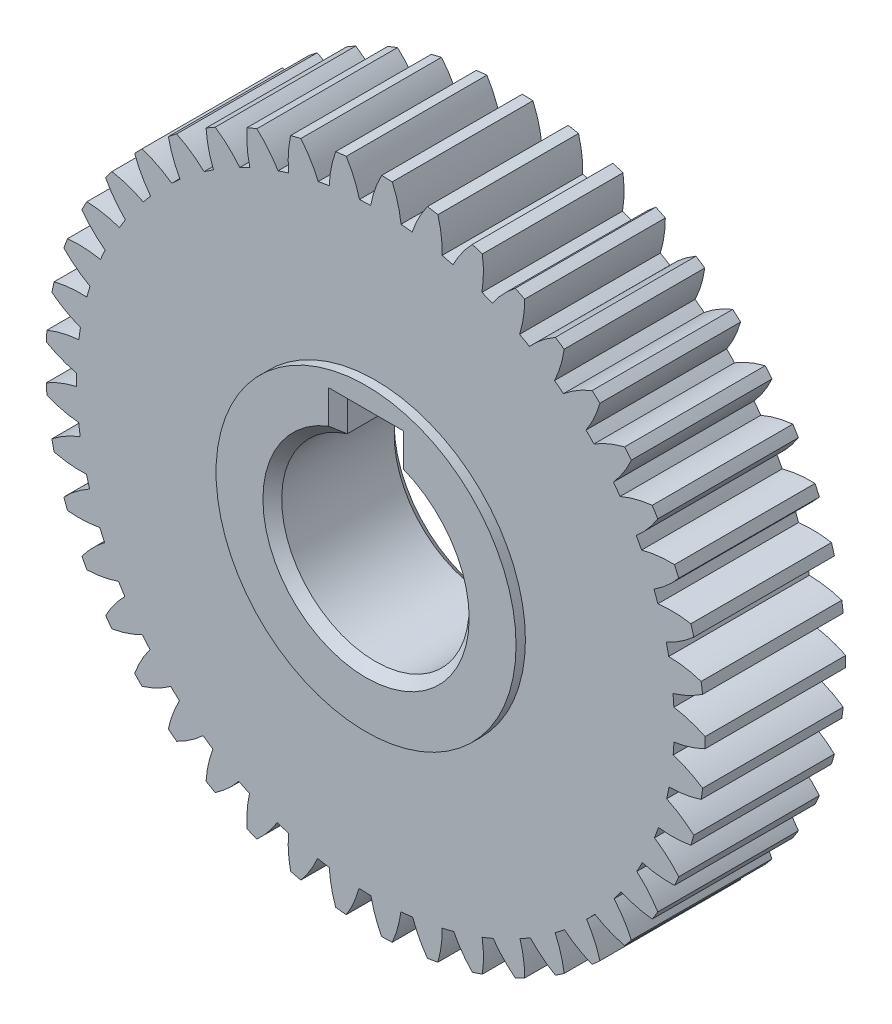
from build123d import *

# Parameters (mm, degrees)
SKETCH1_R           = 31.875
BOSS_EXTRUDE1_DEPTH = 15
BOSS_EXTRUDE2_START = -15
BOSS_EXTRUDE2_DEPTH = 15
CIRPATTERN1_COUNT   = 45
SKETCH3_R           = 16
BOSS_EXTRUDE3_DEPTH = 1
SKETCH5_R           = 10
SKETCH5_W           = 6
SKETCH5_H           = 5.6
CUT_EXTRUDE1_DEPTH  = 53.297227132
SKETCH6_R           = 20
CUT_EXTRUDE2_DEPTH  = 2
CHAMFER1_SIZE       = 1


with BuildPart() as part:
    # Sketch1 → Boss-Extrude1 (new body)
    with BuildSketch(Plane.XY):
        Circle(SKETCH1_R)
    extrude(amount=BOSS_EXTRUDE1_DEPTH)

    # Sketch2 → Boss-Extrude2 (add)
    with BuildSketch(Plane.XY.offset(15).offset(BOSS_EXTRUDE2_START)):
        with BuildLine():
            ThreePointArc((2.731177174, 31.757775367), (2.39625714, 33.517575809), (1.793089986, 35.204365188))
            ThreePointArc((1.793089986, 35.204365188), (1.230207259, 35.228526652), (0.667010267, 35.243688758))
            ThreePointArc((0.667010267, 35.243688758), (-0.052352081, 33.603083127), (-0.50921374, 31.870932311))
            ThreePointArc((-0.50921374, 31.870932311), (1.112421457, 31.855582611), (2.731177174, 31.757775367))
        make_face()
    boss_extrude2 = extrude(amount=BOSS_EXTRUDE2_DEPTH)

    # CirPattern1: Boss-Extrude2 ×45 about axis
    cirpattern1_axis = Axis((0.002916843, 0.083527459, 0), (0, 0, 1))
    for i in range(1, CIRPATTERN1_COUNT):
        add(boss_extrude2.rotate(cirpattern1_axis, i * 360 / CIRPATTERN1_COUNT))

    # Sketch3 → Boss-Extrude3 (add)
    with BuildSketch(Plane.XY.offset(15)):
        Circle(SKETCH3_R)
    extrude(amount=BOSS_EXTRUDE3_DEPTH)

    # Sketch5 → Cut-Extrude1 (cut, through all)
    with BuildSketch(Plane.XY.offset(16)):
        Circle(SKETCH5_R)
        with Locations((0, 10)):
            Rectangle(SKETCH5_W, SKETCH5_H)
    extrude(amount=-CUT_EXTRUDE1_DEPTH, mode=Mode.SUBTRACT)

    # Sketch6 → Cut-Extrude2 (cut)
    with BuildSketch(Plane(origin=(0, 0, 0), x_dir=(-1, 0, 0), z_dir=(0, 0, -1))):
        Circle(SKETCH6_R)
    extrude(amount=-CUT_EXTRUDE2_DEPTH, mode=Mode.SUBTRACT)

    # Chamfer1
    chamfer1_edges = [part.edges().sort_by_distance(p)[0] for p in [
        (-3, 11.169696007, 16),
        (0, 12.8, 16),
        (0, -10, 16),
        (3, 11.169696007, 16),
        (0, -10, 2),
        (3, 11.169696007, 2),
        (-3, 11.169696007, 2),
        (0, 12.8, 2),
    ]]
    chamfer(chamfer1_edges, length=CHAMFER1_SIZE)


solid = part.part
